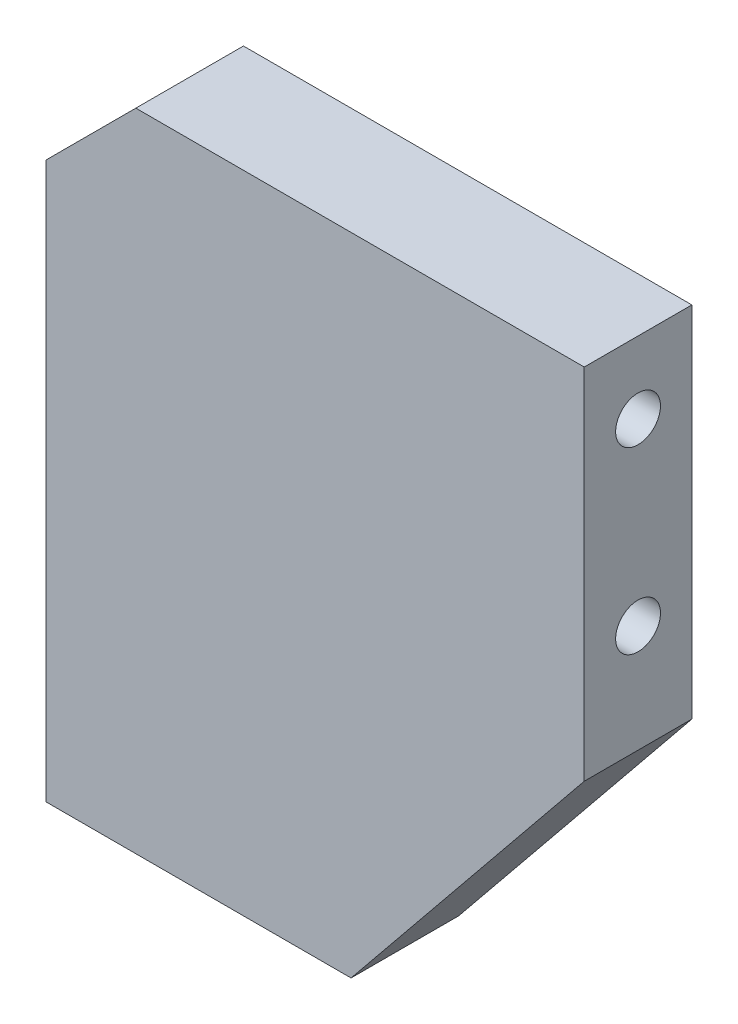
SolidWorks part; units mm, degrees
material "6061-T6 (SS)"
ref_plane "前视基准面" through (0, 0, 0) normal (0, 0, 1) x (1, 0, 0)
ref_plane "上视基准面" through (0, 0, 0) normal (0, 1, 0) x (1, 0, 0)
ref_plane "右视基准面" through (0, 0, 0) normal (1, 0, 0) x (0, 0, -1)
sketch "草图1" plane through (0, 0, 0) normal (0, 0, 1) x (1, 0, 0)
  line L0 (-39.9986, 12) -> (-39.9986, -28)
  line L5 (-99.9986, -60) -> (-99.9986, 12)
  line L6 (-99.9986, 12) -> (-39.9986, 12)
  line L7 (-99.9986, -60) -> (-65.9986, -60)
  line L8 (-65.9986, -60) -> (-39.9986, -28)
  dimension "D1" = 60
  dimension "D2" = 34
  dimension "D3" = 40
  dimension "D4" = 72
extrude "凸台-拉伸1" add sketch "草图1" along normal blind 12
chamfer "倒角1" distance 10 angle 45 1 edges at (-99.9986, 12, 6)
hole_wizard "M6 螺纹孔1" positions "草图3" profile "草图2" tap size "M6" standard "Iso"
sketch "草图3" plane through (-39.9986, 0, 0) normal (1, 0, 0) x (0, 0, -1)
  line L0 (-12, 12) -> (0, 12) construction
  line L1 (0, -28) -> (0, 12) construction
  point P0 (-6, 4)
  point P2 (-6, -16)
  dimension "D1" = 8
  dimension "D2" = 20
  dimension "D3" = 6
sketch "草图2" plane through (-39.9986, 4, 6) normal (0, 1, 0) x (0, 0, -1)
  line L0 (0, 0) -> (0, 14.5022)
  line L1 (0, 14.5022) -> (2.5, 13)
  line L2 (2.5, 13) -> (2.5, 0)
  line L5 (2.5, 0) -> (0, 0)
  line L10 (0, 14.5022) -> (-2.5, 13) construction
  line L11 (0, -6.35) -> (0, 107.95) construction
  dimension "螺纹孔钻头直径" = 5
  dimension "螺纹孔钻头深度" = 13
  dimension "导头角度" = 118
cosmetic thread "孔螺蚊线1" parameters "D1"=13, "D2"=6
cosmetic thread "孔螺蚊线2" parameters "D1"=13, "D2"=6
hole_wizard "M6 螺纹孔2" positions "草图5" profile "草图4" tap size "M6" standard "Iso"
sketch "草图5" plane through (-99.9986, 0, 0) normal (-1, 0, 0) x (0, 0, 1)
  line L0 (0, 12) -> (12, 12) construction
  line L1 (0, 2) -> (0, -60) construction
  point P0 (6, -8)
  point P2 (6, -48)
  dimension "D1" = 20
  dimension "D2" = 40
  dimension "D3" = 6
sketch "草图4" plane through (-99.9986, -8, 6) normal (0, 1, 0) x (0, 0, 1)
  line L0 (0, 0) -> (0, 14.5022)
  line L1 (0, 14.5022) -> (2.5, 13)
  line L2 (2.5, 13) -> (2.5, 0)
  line L5 (2.5, 0) -> (0, 0)
  line L10 (0, 14.5022) -> (-2.5, 13) construction
  line L11 (0, -6.35) -> (0, 107.95) construction
  dimension "螺纹孔钻头直径" = 5
  dimension "螺纹孔钻头深度" = 13
  dimension "导头角度" = 118
cosmetic thread "孔螺蚊线3" parameters "D1"=12, "D2"=6
cosmetic thread "孔螺蚊线4" parameters "D1"=12, "D2"=6
